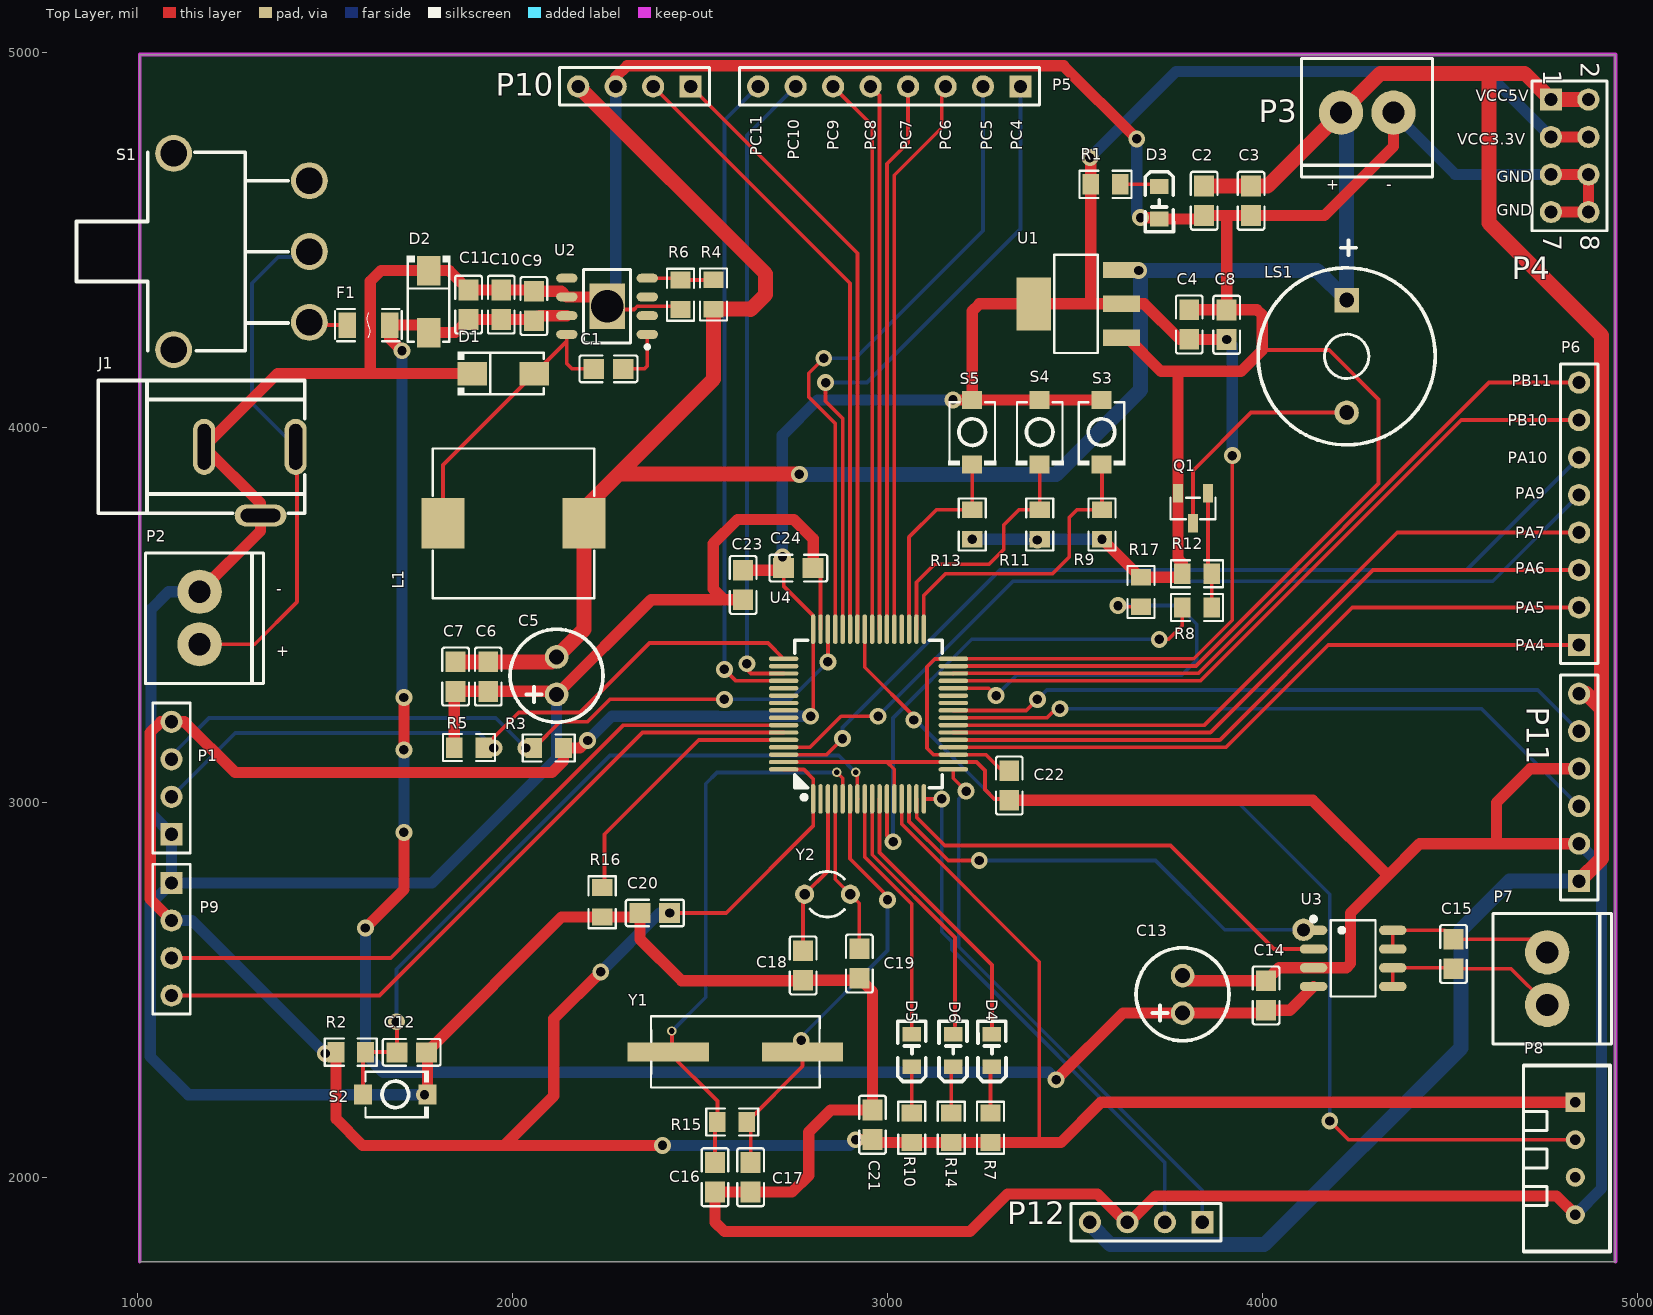
[diagram p0: Top Layer view]
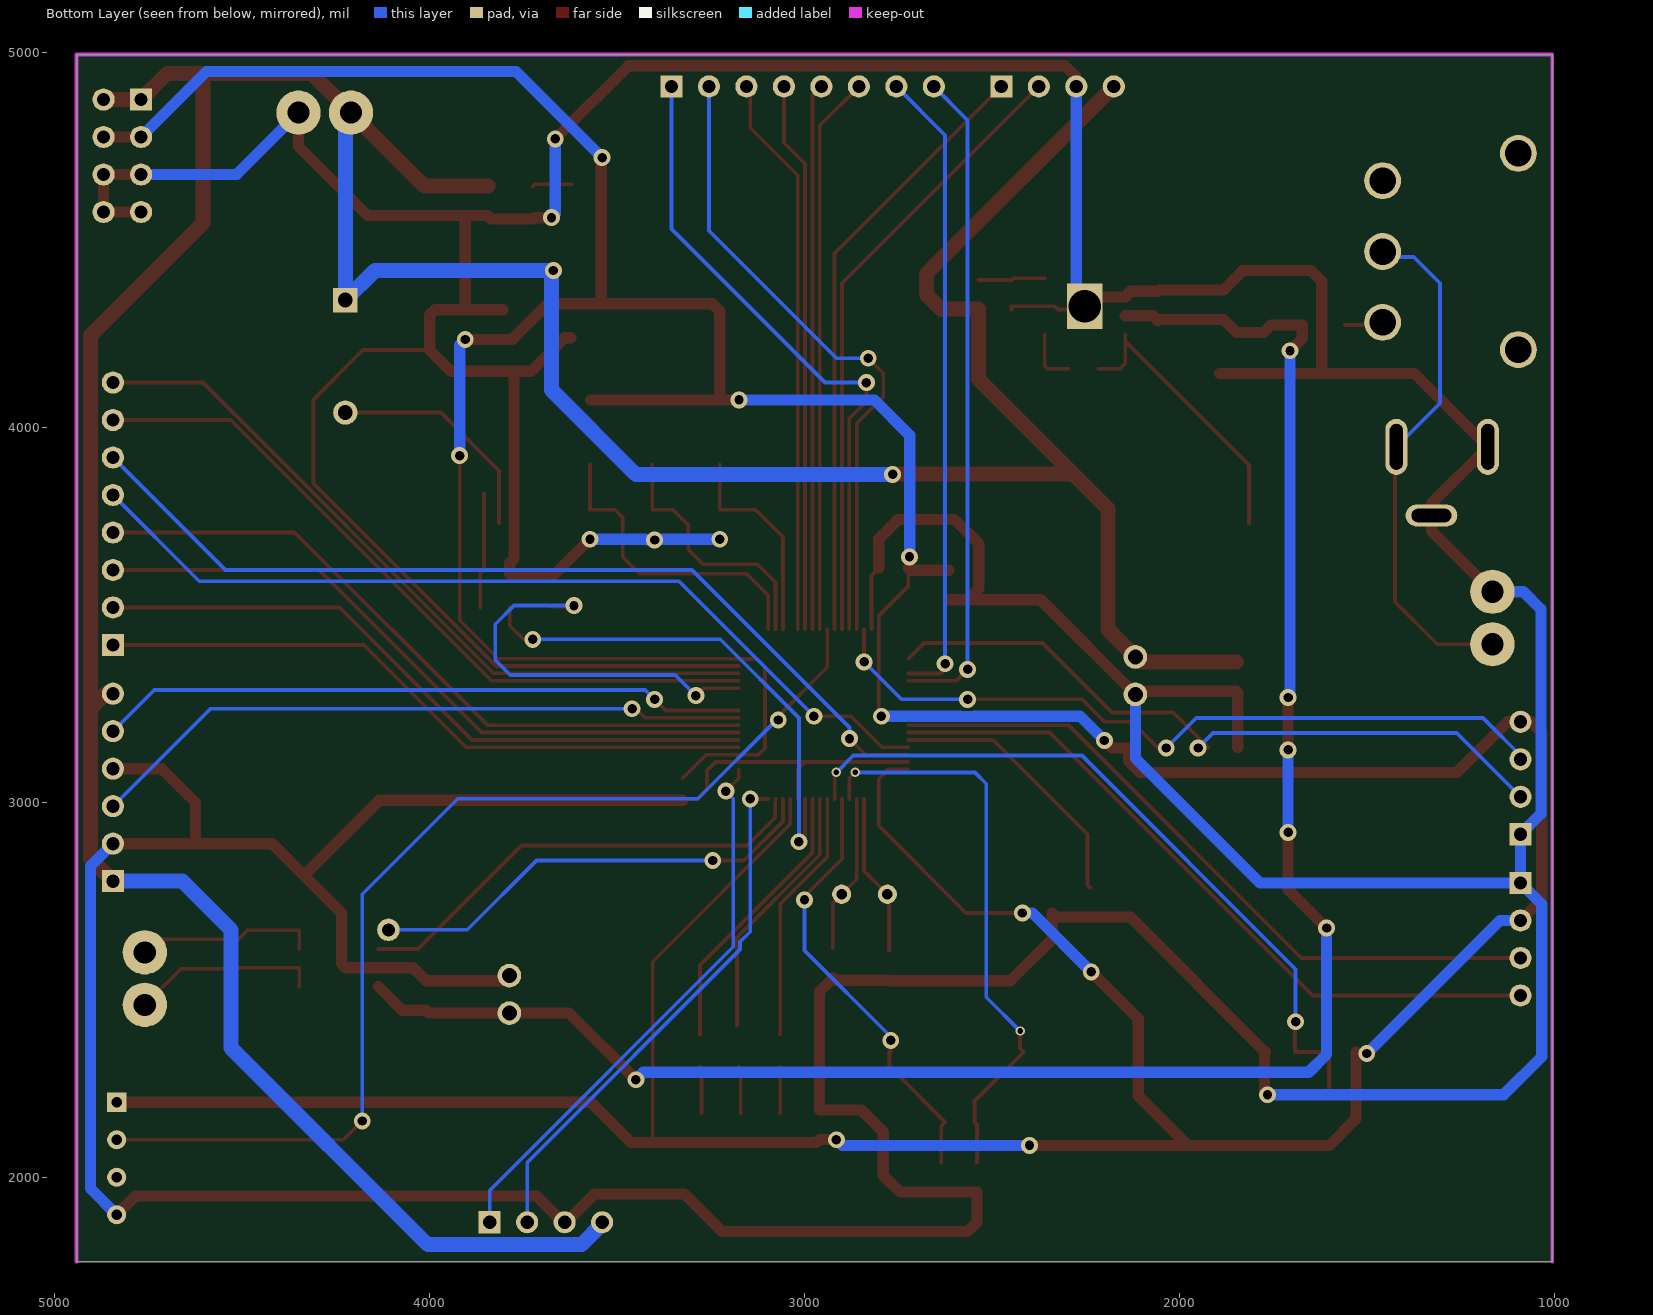
[diagram p1: Bottom Layer view, seen from below]
# Altium PCB MISC82341.PcbDoc
Units mil, origin at the board's own origin, x right, y up, seen from the top; angles counter-clockwise.
Board outline 3937.01 x 3220 mil, 2 copper layers (Top Layer, Bottom Layer); 75 components, 60 nets, 265 pads, 53 vias.

## Layer stack, top to bottom (the 12.6 mil dielectric is the usual default, probably not edited)
Top Solder: solder mask 0.4, Solder Resist, Dk 3.5
Top Layer: signal copper 1.4
Dielectric 1: dielectric 12.6, FR-4, Dk 4.8
Bottom Layer: signal copper 1.4
Bottom Solder: solder mask 0.4, Solder Resist, Dk 3.5

## Board outline
1005,1775 1005,4995 4942.01,4995 4942.01,1775

## Design rules (kind name [scope] priority, off if disabled: settings)
Clearance [All] p1: gap=8 ignorepadtopadclearanceinfootprint=FALSE except(7: SMDPad-SMDPad; 10: Arc-Fill Arc-Poly Arc-Region Track-Fill Track-Poly Track-Region THPad-Fill THPad-Poly THPad-Region Via-Fill Via-Poly Via-Region Fill-Fill Fill-Poly Fill-Region Poly-Poly Poly-Region Region-Region; 13: SMDPad-Fill SMDPad-Poly SMDPad-Region)
HoleSize [All] p1: absolutevalues=TRUE maxlimit=200 minlimit=1 maxpercent=80.000 minpercent=20.000
PolygonConnect [All] p1: connectstyle=Relief reliefconductorwidth=10 reliefentries=4 polygonreliefangle="90 Angle" airgapwidth=10
RoutingVias [All] p1: holewidth=20 width=30 viastyle="Through Hole" minholewidth=12 minwidth=24 maxholewidth=28 maxwidth=50
SolderMaskExpansion [All] p1: expansion=4
Width [All] p1: maxlimit=120 minlimit=8 preferedwidth=10
29 further rules are at their usual default settings.

## Components (designator, comment, footprint, x,y, rotation, side; value= is the part's Value field where it differs from the comment)
C1 "0.01uF" C0805 2255.63,4156.65 r180 top
C2 "10uF" C0805 3845,4605 r90 top
C3 "0.1uF" C0805 3970,4605 r90 top
C4 "10uF" C0805 3805,4275 r270 top
C5 "330uF/16V" 220uF 2110,3335 r90 top
C6 "0.1uF" C0805 1935,3335.63 r90 top
C7 "0.01uF" C0805 1847.84,3335.63 r90 top
C8 "0.1uF" C0805 3905,4274.37 r270 top
C9 "10uF/25V" C0805 2056.77,4324.17 r270 top
C10 "10uF/25V" C0805 1969.61,4327.91 r270 top
C11 "0.01uF" C0805 1882.45,4327.91 r270 top
C12 "0.1uF" C0805 1730.63,2333.33 r0 top
C13 "220uF/16V" 220uF 3780,2485 r90 top
C14 "0.01uF" C0805 4010,2485 r90 top
C15 "0.01uF" C0805 4510,2595.63 r90 top
C16 "22pF" C0805 2540,2000 r270 top
C17 "22pF" C0805 2635,2000 r270 top
C18 "15pF" C0805 2775,2565 r90 top
C19 "15pF" C0805 2925,2570 r270 top
C20 "0.1uF" C0805 2379.37,2705 r180 top
C21 "0.1uF" C0805 2960,2140 r90 top
C22 "0.1uF" C0805 3325,3045 r270 top
C23 "0.1uF" C0805 2615,3580 r270 top
C24 "0.1uF" C0805 2762.37,3625 r0 top
D1 "SS54" SMA 1975,4145 r0 top
D2 "SMBJ12A" SMA 1776.6,4336.74 r270 top
D3 "LED0" LED0805-RD_RED 3725,4600 r270 top
D4 "LED0" LED0805-RD_RED 3278.7,2338.31 r90 top
D5 "LED0" LED0805-RD_RED 3065,2338.31 r90 top
D6 "LED0" LED0805-RD_RED 3175,2338.31 r90 top
F1 "3A/16V" C70065 1611.93,4269.92 r0 top
J1 "DC-jack3" SANJIAO 1168.34,3957.44 r90 top
L1 "Inductor" DIANGAN 2005,3735 r180 top
LS1 "Speaker" BZ 4235,3805 r270 top
P1 "Header 4" HDR1X4 1090,2915 r90 top
P2 "Header 2" KF350 1165,3486.88 r180 top
P3 "Header 2" KF350 4275,4840 r90 top
P4 "Header 4X2" HDR2X4 4770,4875 r270 top
P5 "Header 8" HDR1X8 3355,4910 r180 top
P6 "Header 8" HDR1X8 4845,3420 r90 top
P7 "Header 2" KF350 4760,2525 r180 top
P8 "DHT11" DHT11 2528.78,-2097.7 r270 top
P9 "Header 4" HDR1X4 1090,2785 r270 top
P10 "HC-06" HDR1X4 2475,4910 r180 top
P11 "GP2Y1010AU0F" HDR1X6 4845,2790 r90 top
P12 "JW01" HDR1X4 3840,1880 r180 top
Q1 "NPN" QNPN 3815,3790 r90 top
R1 "10K" R0805 3580,4650 r180 top
R2 "10K" R0805 1566.41,2335.08 r180 top
R3 "10K" R0805 2094.58,3146.22 r180 top
R4 "10K" R0805 2534.78,4353.54 r270 top
R5 "10K" R0805 1885,3145 r0 top
R6 "3.16K" R0805 2449.01,4355.93 r90 top
R7 "10K" R0805 3273.78,2130.47 r270 top
R8 "1K" R0805 3827.19,3518.78 r0 top
R9 "10K" R0805 3571.06,3740 r270 top
R10 "10K" R0805 3063.78,2130.47 r270 top
R11 "10K" R0805 3405,3740 r270 top
R12 "10K" R0805 3827.19,3608.78 r0 top
R13 "10K" R0805 3225,3740 r270 top
R14 "10K" R0805 3168.78,2130.47 r270 top
R15 "1M" R0805 2584.07,2148.58 r180 top
R16 "10K" R0805 2240,2735 r90 top
R17 "10K" R0805 3675,3560 r270 top
S1 "SW-SPDT" SW-TH 1127.09,4463.54 r90 top
S2 "SW-PB" KAIGUAN 1685,2220 r0 top
S3 "SW-PB" KAIGUAN 3570,3990 r270 top
S4 "SW-PB" KAIGUAN 3405,3990 r270 top
S5 "SW-PB" KAIGUAN 3225,3990 r270 top
U1 "AMS1117" SOT-89 4700.81,4809.72 r0 top
U2 "TPS5450" CYF-SOIC-H 2252.01,4323.54 r180 top
U3 "RZ7889" SOP-8 4250,2580 r270 top
U4 "stm32f103r" LQFP-64 2945,3245 r0 top
Y1 "8MHz" JINGZHEN 2590,2335 r180 top
Y2 "32.768KHz" R38 2840,2755 r270 top

## Footprints (in the part's own frame and the unit in brackets; to place one, negate y for a bottom-side part, rotate by r counter-clockwise, add the part's x,y. Pads: shape width x height; smd on the part's side, far side on the other; paste and mask are expansions set on the pad)
220uF [mm]
  round 1.6 hole 1: 1(-1.193,-0.185) 2(1.347,-0.185)
  silkscreen extent -3.07,-3.33 3.23,2.96
BZ [mm]
  rect 1.65x1.65 hole 1: 1(-13.589,-0.254)
  round 1.65 hole 1: 2(-5.969,-0.254)
  silkscreen extent -17.65,-6.25 -3.78,5.75
C0805 [mm]
  rect 1.41x1.35 smd: 1(-1,0) 2(1,0)
  silkscreen extent -1.96,-0.9 1.96,0.9
C70065 [mil]
  rect 46.85x68.03 smd: 1(-53.62,3.62) 2(60.16,3.62)
  silkscreen extent -86,-39 93,47
CYF-SOIC-H [mm] "SOIC, 8-Leads, Body 4.90x3.90mm, Pitch 1.27mm, Thermal Pad 3.10x2.40mm, IPC Medium Density"
  oval 1.45x0.6 smd: 1(-2.725,1.905) 2(-2.725,0.635) 3(-2.725,-0.635) 4(-2.725,-1.905) 5(2.725,-1.905) 6(2.725,-0.635) 7(2.725,0.635) 8(2.725,1.905)
  rect 2.4x3.1 hole 2.2: 9(0,0)
  silkscreen extent -2.85,-2.5 1.6,2.88, body extent -2,-2.5 2,2.5, height 1.7
DHT11 [mil]
  rect 51x51 hole 28: 1(-4297.7,2306.22)
  round 51 hole 28: 2(-4197.7,2306.22) 3(-4097.7,2306.22) 4(-3997.7,2306.22)
  silkscreen extent -4396,2168 -3899,2399
DIANGAN [mm]
  rect 2.924x3.42 smd: 1(4.844,-0.241) 2(-4.712,-0.241)
  silkscreen extent -5.41,-5.32 5.54,4.84
HDR1X4 [mm] "Connector; Header; 4 Position"
  rect 1.5x1.5 hole 0.9: 1(0,0)
  round 1.5 hole 0.9: 2(2.54,0) 3(5.08,0) 4(7.62,0)
  silkscreen extent -1.27,-1.27 8.89,1.27
HDR1X6 [mm] "Connector; Header; 6 Position"
  rect 1.5x1.5 hole 0.9: 1(0,0)
  round 1.5 hole 0.9: 2(2.54,0) 3(5.08,0) 4(7.62,0) 5(10.16,0) 6(12.7,0)
  silkscreen extent -1.27,-1.27 13.97,1.27
HDR1X8 [mm] "Connector; Header; 8 Position"
  rect 1.5x1.5 hole 0.9: 1(0,0)
  round 1.5 hole 0.9: 2(2.54,0) 3(5.08,0) 4(7.62,0) 5(10.16,0) 6(12.7,0) 7(15.24,0) 8(17.78,0)
  silkscreen extent -1.27,-1.27 19.05,1.27
HDR2X4 [mm] "Connector; Header; 4x2 Position"
  rect 1.5x1.5 hole 0.9: 1(0,0)
  round 1.5 hole 0.9: 2(0,2.54) 3(2.54,0) 4(2.54,2.54) 5(5.08,0) 6(5.08,2.54) 7(7.62,0) 8(7.62,2.54)
  silkscreen extent -1.27,-1.27 8.89,3.81
JINGZHEN [mm]
  rect 5.5x1.3 smd: 1(-4.665,0.013) 2(4.441,0.013)
  silkscreen extent -5.83,-2.4 5.6,2.43
KAIGUAN [mm]
  rect 1.23x1.36 smd: 1(-2.13,0.027) 2(2.24,0.027)
  silkscreen extent -1.97,-1.59 2.31,1.64
KF350 [mm]
  round 3 hole 1.5: 1(0,-1.905) 2(0,1.651)
  silkscreen extent -4.34,-4.55 3.68,4.32
LED0805-RD_RED [mm]
  rect 1x1.25 smd: 1(-1.1,0) 2(1.1,0)
  silkscreen extent -2.1,-0.95 1.98,0.96
LQFP-64 [mm]
  oval 0.3x2 smd: 1(-3.639,-5.988) 2(-3.139,-5.988) 3(-2.639,-5.988) 4(-2.139,-5.988) 5(-1.639,-5.988) 6(-1.139,-5.988) 7(-0.639,-5.988) 8(-0.139,-5.988) 9(0.361,-5.988) 10(0.861,-5.988) 11(1.361,-5.988) 12(1.861,-5.988) 13(2.361,-5.988) 14(2.861,-5.988) 15(3.361,-5.988) 16(3.861,-5.988) 33(3.861,5.512) 34(3.361,5.512) 35(2.861,5.512) 36(2.361,5.512) 37(1.861,5.512) 38(1.361,5.512) 39(0.861,5.512) 40(0.361,5.512) 41(-0.139,5.512) 42(-0.639,5.512) 43(-1.139,5.512) 44(-1.639,5.512) 45(-2.139,5.512) 46(-2.639,5.512) 47(-3.139,5.512) 48(-3.639,5.512)
  oval 2x0.3 smd: 17(5.861,-3.988) 18(5.861,-3.488) 19(5.861,-2.988) 20(5.861,-2.488) 21(5.861,-1.988) 22(5.861,-1.488) 23(5.861,-0.988) 24(5.861,-0.488) 25(5.861,0.012) 26(5.861,0.512) 27(5.861,1.012) 28(5.861,1.512) 29(5.861,2.012) 30(5.861,2.512) 31(5.861,3.012) 32(5.861,3.512) 49(-5.639,3.512) 50(-5.639,3.012) 51(-5.639,2.512) 52(-5.639,2.012) 53(-5.639,1.512) 54(-5.639,1.012) 55(-5.639,0.512) 56(-5.639,0.012) 57(-5.639,-0.488) 58(-5.639,-0.988) 59(-5.639,-1.488) 60(-5.639,-1.988) 61(-5.639,-2.488) 62(-5.639,-2.988) 63(-5.639,-3.488) 64(-5.639,-3.988)
  silkscreen extent -4.89,-6.03 5.11,4.76
QNPN [mm]
  rect 1.25x0.7 smd: 1(-1.143,0) 2(0.889,-1.016) 3(0.889,1.016)
  silkscreen extent -0.88,-1.52 0.57,1.53
R38 [mm] "Crystal, Thru-Hole; 2 Leads; Body 3.1 x 8.2 mm (Dia.xH)"
  round 1.3 hole 0.7: 1(0,1.55) 2(0,-1.55)
  silkscreen extent -1.55,-1.19 1.55,1.17
R0805 [mil]
  rect 44.59x54.21 smd: 1(-40.93,1.22) 2(37.81,1.22)
  silkscreen extent -71,-35 68,37
SANJIAO [mm]
  oval 3.8x1.5 hole 0.9 slot 3.1 at 0 deg: 1(-0.226,-6.422) 2(-0.226,-0.222)
  oval 1.5x3.5 hole 0.9 slot 2.7 at 90 deg: 3(-4.876,-4.044)
  silkscreen extent -4.73,-7.04 4.27,6.96
SMA [mm]
  rect 2x1.593 smd: 1(-2.087,-0.023) 2(2.113,-0.023)
  silkscreen extent -3.09,-1.5 2.74,1.45
SOP-8 [mm]
  oval 0.63x1.865 smd: 1(-2.004,-2.878) 2(-0.734,-2.878) 3(0.536,-2.878) 4(1.806,-2.878) 5(1.806,2.487) 6(0.536,2.487) 7(-0.734,2.487) 8(-2.004,2.487)
  silkscreen extent -2.92,-3.03 2.48,1.33
SOT-89 [mm]
  rect 2.5x1.1 smd: 1(-27.355,-14.485) 2(-27.355,-12.185) 3(-27.355,-9.885)
  rect 2.34x3.6 smd: 2(-33.294,-12.185)
  silkscreen extent -31.9,-15.51 -28.95,-8.86
SW-TH [mm]
  round 2.5 hole 1.8: 1(-4.647,-8.402) 2(0.153,-8.402) 3(4.953,-8.402) 4(-6.497,0.798) 5(6.803,0.798)
  silkscreen extent -6.58,-6.98 6.88,7.37

## Part data
C1 C2 C3 C4 C5 C6 C7 C8 C9 C10 C11 C12 C13 C14 C15 C16 C17 C18 C19 C20 C21 C22 C23 C24: library part Cap, "Capacitor"
D1 D2: library part "D Schottky", "Schottky Diode"
D3 D4 D5 D6: "Typical INFRARED GaAs LED"
F1: library part "Fuse 1", "Fuse"
LS1: "Loudspeaker"
P1 P9: "Header, 4-Pin"
P2 P3 P7: "Header, 2-Pin"
P4: "Header, 4-Pin, Dual row"
P5 P6: "Header, 8-Pin"
P10 P12: library part "Header 4", "Header, 4-Pin"
P11: library part "Header 6", "Header, 6-Pin"
R1 R2 R3 R4 R5 R6 R7 R8 R9 R10 R11 R12 R13 R14 R15 R16 R17: library part Res2, "Resistor"
S1: "SPDT Subminiature Toggle Switch, Right Angle Mounting, Vertical Actuation"
S2 S3 S4 S5: "Switch"
Y1 Y2: library part XTAL, "Crystal Oscillator"

## Free pads (board coordinates)
  round 60 hole 35: 3(4110,2660)

## Via types
v1: diameter 45, hole 25, Top Layer to Bottom Layer, 50 vias
v2: diameter 25, hole 15, Top Layer to Bottom Layer, 3 vias

## Nets (pads, with @x,y where several pads share a name; then routed paths per layer and width w, separated by ;. In a path a pad name is that pad's centre, name@x,y a point inside that pad or via, vN(x,y) a via of type N, cw(c..) or ccw(c..) an arc to the next point about the centre after c; other vN are vias at no path point)
B: D4.2 U4.10 | length 751.8
  Top Layer w10: U4.10 2978.91,2866.09 3278.7,2566.3 D4.2
BEEP: R8.1 U4.11 | length 1373.1
  Top Layer w10: U4.11 2998.59,2911.41 v1(3015,2895) ; v1(3725,3435) 3750,3435 3786.26,3471.26 R8.1
  Bottom Layer w10: v1(3015,2895) 3015,3225 3225,3435 v1(3725,3435)
"CAN RX": P5.1 U4.44 | length 1746.9
  Top Layer w10: v1(2835,4120) 2835,4070 2880.48,4024.52 U4.44
  Bottom Layer w10: v1(2835,4120) 2945.48,4120 3355,4529.52 P5.1
"CAN TX": P5.2 U4.45 | length 1719.7
  Top Layer w10: v1(2830,4185) 2790,4145 2790,4081.74 2860.8,4010.94 U4.45
  Bottom Layer w10: v1(2830,4185) 2915,4185 3255,4525 P5.2
DATA: P8.2 U4.41 | length 2893.5
  Top Layer w10: U4.41 2939.54,3360.46 3080,3220 v1(3070,3220) ; v1(4180,2150) 4230,2100 P8.2
  Bottom Layer w10: v1(3070,3220) 3075,3220 3285,3010 3925,3010 4180,2755 v1(4180,2150)
"DC IN": C9.2 C10.2 C11.2 C13.1 C14.1 D2.2 F1.2 U2.7 U3.4 | length 5155.2
  Top Layer w30: v1(1607.35,2665) 1710,2767.65 v1(1710,2920) ; v1(1705,4205) 1672.09,4237.91 F1.2 1755.7,4273.54 D2.2 1847.45,4253.54 C11.2 C10.2 2053.03,4288.54 C9.2 2070.51,4298.54 U2.7 ; v1(1710,3140) v1(1710,3280) ; v1(3450,2260) 3628.02,2438.02 C13.1 4002.39,2438.02 C14.1 4073.46,2445.63 U3.4
  Bottom Layer w30: v1(1607.35,2665) 1607.35,2327.65 1655,2280 3430,2280 v1(3450,2260) ; v1@1705,3290 v1(1705,4205) ; v1(1710,2920) v1(1710,3140)
G: D6.2 U4.9 | length 695.7
  Top Layer w10: U4.9 2959.22,2860.33 3180,2639.54 3180,2405
GND: C2.1 C3.1 C4.1 C5.1 C6.1 C7.1 C8.1 C9.1 C10.1 C11.1 C12.2 C13.2 C14.2 C16.2 C17.2 C18.1 C19.2 C20.2 C21.2 C22.2 C23.2 C24.2 D1.1 D2.1 D3.2 J1.2 J1.3 P1.1 P2.1 P3.1 P4.5 P4.6 P4.7 P4.8 P8.4 P9.1 P10.3 P11.2 P11.4 P12.3 Q1.3 R5.1 R6.1 R9.2 R11.2 R12.1 R13.2 R16.1 R17.1 S2.2 U1.1 U2.6 U2.9 U3.3 U4.12 U4.18 U4.31 U4.47 U4.63 | length 25294.4
  Top Layer w10: U2.9 2260.55,4315 2323.94,4315 2332.28,4323.35 2447.78,4323.35 R6.1 ; U4.63 2999.03,3107.69 ; C24.2 2821.43,3605.31 U4.47 ; U4.12 3018.28,3088.44 2999.03,3107.69 ; U4.31 3823.13,3363.59 4310,3850.46 4310,4075 4178.35,4206.65 4000,4206.65 ; C22.2 3321.36,3009.27 3285,3009.27 3260,3034.27 3260,3085 3237.31,3107.69 U4.18 2999.03,3107.69
  Top Layer w30: P2.1 1327.57,3724.45 J1.3 1327.57,3798.06 J1.2 1372.65,4144.1 1620,4144.1 ; S2.2 1773.2,2330.13 C12.2 2130.74,2694.07 R16.1 2329.07,2694.07 C20.2 2340,2635 2450.63,2524.37 2773.74,2524.37 C18.1 2920,2525.63 C19.2 2960,2495.63 C21.2 2848.74,2179.37 2790,2120.63 2790,2005 2745.63,1960.63 C17.2 C16.2 2540,1880 2565,1855 3220,1855 3320,1955 3560,1955 3640,1875 3715,1950 4785,1950 P8.4 ; R5.1 1844.07,3292.49 C7.1 C6.1 2109.05,3296.26 C5.1 2369.9,3540.63 2564.37,3540.63 ; D1.1 1620,4144.1 ; U2.9 2227.01,4348.54 U2.6 2129.73,4363.54 C9.1 2053.03,4367.28 C10.1 C11.1 1830.83,4418.9 D2.1 1648.9,4418.9 1620,4390 1620,4144.1 ; P10.3 2275,4935 2305,4965 3470,4965 v1@3660,4775 ; C23.2 2564.37,3540.63 ; C24.2 2801.74,3703.26 2750,3755 2600,3755 2535,3690 2535,3570 2564.37,3540.63 ; C22.2 4134.37,3005.63 4335,2805 ; v1(3572.29,3702.19) 3673.55,3600.93 R17.1 3777.19,3600.93 R12.1 3786.26,3638.74 3775,3650 Q1.3 3775,4145 3770,4150 ; U1.1 3640.55,4239.45 3730,4150 3770,4150 ; v1(3675,4560) 3721.7,4560 D3.2 3836.06,4556.69 C2.1 3900,4565.63 ; C13.2 3800.94,2524.37 C14.2 4044.51,2558.88 U3.3 4223.88,2558.88 4235,2570 4235,2705 4335,2805 ; C4.1 C8.1@3905,4314.37 ; P3.1 4350,4750 4165.63,4565.63 C3.1 3900,4565.63 ; P4.7 P4.8 P4.6 P4.5 ; P11.2 4625,2890 ; P11.4 4715,3090 4625,3000 4625,2890 ; 3770,4150 3943.35,4150 4000,4206.65 4000,4300 3985,4315 3984.37,4314.37 C8.1@3905,4314.37 ; 3900,4565.63 3905,4560.63 C8.1@3905,4314.37 ; 4335,2805 4420,2890 4625,2890
  Bottom Layer w30: P9.1@1080,2785 1090,2795 P1.1 1035,2970 1035,3515 1081.88,3561.88 P2.1 ; v1(1765,2220) 1135,2220 1033,2322 1033,2728 P9.1 1785,2785 2117.29,3117.29 C5.1 ; U2.9 2275,4346.53 P10.3 ; v1(3226.22,3702.19) v1@3400,3702.19 ; v1(3400,3700) 3422.81,3700 3425,3702.19 v1(3572.29,3702.19) ; v1(3665,4770) 3665,4570 v1(3675,4560) ; P3.1 4515,4675 P4.5 ; P8.4 4905,1970 4905,2830 P11.2
NetC1_1: C1.1 U2.1 | length 151.7
  Top Layer w10: C1.1 2351.65,4156.65 2359.29,4164.29 U2.1
NetC1_2: C1.2 D1.2 L1.1 U2.8 | length 778.5
  Top Layer w10: L1.1 1814.28,3900.18 D1.2 2144.73,4230.62 ; U2.8 2144.73,4230.62 ; C1.2 2158.35,4156.65 2144.73,4170.27 2144.73,4230.62
NetC15_1: C15.1 P7.2 U3.5 U3.6 | length 503
  Top Layer w10: U3.5 U3.6 4507.38,2558.88 C15.1 4663.74,2556.26 P7.2
NetC15_2: C15.2 P7.1 U3.7 U3.8 | length 486.5
  Top Layer w10: U3.7 U3.8 4486.12,2658.88 C15.2 4725,2635 P7.1
NetC16_1: C16.1 R15.2 U4.5 Y1.2 | length 1548.4
  Top Layer w10: v2(2425,2390) 2425,2344.3 Y1.2 2546.26,2203.39 R15.2 2540,2141.1 C16.1 ; v2(2865,3080) 2880.48,3064.52 U4.5
  Bottom Layer w10: v2(2425,2390) 2515,2480 2515,3050 2545,3080 v2(2865,3080)
NetC17_1: C17.1 R15.1 U4.6 Y1.1 | length 1172.7
  Top Layer w10: C17.1 2635,2137.36 R15.1 2773.67,2296.03 Y1.1 2770.52,2334.48 2770,2335 v1(2770,2365) ; U4.6 2900.17,2849.83 v1@3005,2745
  Bottom Layer w10: v1(2770,2365) 2770,2375 3000,2605 v1(3000,2740)
NetC18_2: C18.2 U4.3 Y2.2 | length 432.3
  Top Layer w10: C18.2 2775,2751.02 Y2.2 2841.11,2817.13 U4.3
NetC19_1: C19.1 U4.4 Y2.1 | length 426.5
  Top Layer w10: U4.4 2860.8,2795.22 Y2.1 2925,2731.02 C19.1
NetD3_1: D3.1 R1.1 | length 106.3
  Top Layer w10: R1.1 3719.54,4648.78 D3.1
NetD4_1: D4.1 R7.1 | length 125.1
  Top Layer w10: R7.1 3275,2291.3 D4.1
NetD5_1: D5.1 R10.1 | length 123.6
  Top Layer w10: R10.1 D5.1
NetD6_1: D6.1 R14.1 | length 125.7
  Top Layer w10: R14.1 3170,2290 D6.1
NetF1_1: F1.1 S1.1 | length 103.4
  Top Layer w10: S1.1 1464.91,4273.54 F1.1
NetJ1_1: J1.1 P2.2 S1.2 | length 1394.5
  Top Layer w10: P2.2 1311.88,3421.88 1425,3535 1425,3944.73 J1.1
  Bottom Layer w10: J1.1 1305,4064.73 1305,4385 1375,4455 1443.31,4455 S1.2
NetLS1_2: LS1.2 Q1.1 | length 614.2
  Top Layer w10: Q1.1 3815,3885 3970,4040 LS1.2
NetQ1_2: Q1.2 R8.2 R12.2 | length 309.1
  Top Layer w10: Q1.2 3855,3620 R12.2 R8.2
NetR4_1: R4.1 R6.2 U2.4 | length 179
  Top Layer w10: U2.4 2442.98,4398.54 R6.2 2535.27,4393.74 R4.1
NetR16_2: R16.2 U4.60 | length 727.1
  Top Layer w10: R16.2 2245,2779.03 2245,2915 2496.74,3166.74 U4.60
NetR17_2: R17.2 U4.28 | length 1084.8
  Top Layer w10: U4.28 3270.46,3304.54 v1(3290,3285) ; v1(3615,3525) 3617.81,3522.19 R17.2
  Bottom Layer w10: v1(3290,3285) 3345,3340 3785,3340 3825,3380 3825,3475 3775,3525 v1(3615,3525)
PA0: pad.3 U3.1 U4.14 | length 1227.1
  Top Layer w10: U4.14 3057.65,2949.37 3162.02,2845 v1@3240,2845
  Bottom Layer w10: v1(3245,2845) 3715,2845 3900,2660 pad.3
PA1: U3.2 U4.15 | length 1253.9
  Top Layer w10: U4.15 3078.11,3008.49 3078.11,2959.6 3152.71,2885 3755,2885 4031.12,2608.88 U3.2
PA2: P12.2 U4.16 | length 1428.7
  Top Layer w10: U4.16 v1(3145,3009.27)
  Bottom Layer w10: v1(3145,3009.27) 3145,2655 3172,2628 3172,2607.54 3740,2039.54 P12.2 P12.2@3740,1875
PA3: P12.1 U4.17 | length 1504.7
  Top Layer w10: U4.17 3175.75,3064.25 v1(3210,3030)
  Bottom Layer w10: v1(3210,3030) 3190,3010 3190,2615 3840,1965 P12.1 P12.1@3840,1875
PA4: P6.1 U4.20 | length 1782.3
  Top Layer w10: U4.20 3902.84,3147.06 4175.78,3420 P6.1
PA5: P6.2 U4.21 | length 1815.6
  Top Layer w10: U4.21 3886.74,3166.74 4240,3520 P6.2
PA6: P6.3 U4.22 | length 1848.8
  Top Layer w10: U4.22 3861.43,3186.43 4295,3620 P6.3
PA7: P6.4 U4.23 | length 1882.1
  Top Layer w10: U4.23 3846.11,3206.11 4360,3720 P6.4
PA9: P10.1 U4.42 | length 1632.3
  Top Layer w10: P10.1 2919.85,4465.15 U4.42
PA10: P10.2 U4.43 | length 1665.5
  Top Layer w10: P10.2 2900.17,4384.83 U4.43
PB6: P9.3 U4.58 | length 1900.3
  Top Layer w10: P9.3@1080,2585 P9.3 1675,2585 2296.11,3206.11 U4.58
PB7: P9.4 U4.59 | length 1933.5
  Top Layer w10: P9.4@1080,2485 P9.4 1645,2485 2346.43,3186.43 U4.59
PB8: P6.5 U4.61 | length 2400.7
  Top Layer w10: U4.61 2793.49,3147.06 2876.43,3230 v1(2975,3230)
  Bottom Layer w10: v1(2975,3230) 3335,3590 4615,3590 P6.5
PB9: P6.6 U4.62 | length 2467.9
  Top Layer w10: U4.62 2837.37,3127.37 v1(2880,3170)
  Bottom Layer w10: v1(2880,3170) 2880,3200 3300,3620 4545,3620 P6.6
PB10: P6.7 U4.29 | length 1957.5
  Top Layer w10: U4.29 3834.68,3324.22 4530.46,4020 P6.7
PB11: P6.8 U4.30 | length 1990.7
  Top Layer w10: U4.30 3176.52,3344.68 3829.68,3344.68 4605,4120 P6.8
PB12: R9.1 S3.2 U4.33 | length 843
  Top Layer w10: U4.33 3097.02,3552.02 3155,3610 3440,3610 3485,3655 3485,3760 3505.93,3780.93 R9.1 3572.29,3900.58 S3.2
PB13: R11.1 S4.2 U4.34 | length 693.4
  Top Layer w10: U4.34 3077.33,3587.33 3125,3635 3270,3635 3310,3675 3310,3740 3350.93,3780.93 R11.1 3406.22,3901.64 S4.2
PB14: R13.1 S5.2 U4.35 | length 565.5
  Top Layer w10: U4.35 3057.65,3707.65 3130.93,3780.93 R13.1 3226.22,3901.64 S5.2
PC4: P11.3 U4.24 | length 1787
  Top Layer w10: U4.24 3425.8,3225.8 3450,3250 v1(3460,3250)
  Bottom Layer w10: v1(3460,3250) 4585,3250 P11.3
PC5: P11.5 U4.25 | length 1737.4
  Top Layer w10: U4.25 3370.48,3245.48 v1(3400,3275)
  Bottom Layer w10: v1(3400,3275) 3425,3300 4735,3300 P11.5
PC6: P5.3 U4.37 | length 1504.6
  Top Layer w10: U4.37 3018.28,4673.28 3145,4800 3145,4900 P5.3
PC7: P5.4 U4.38 | length 1471.4
  Top Layer w10: U4.38 2998.59,4703.59 3055,4760 P5.4
PC8: P5.5 U4.39 | length 1457.9
  Top Layer w10: P5.5 2978.91,4886.09 U4.39
PC9: P5.6 U4.40 | length 1491.2
  Top Layer w10: P5.6 2959.22,4805.78 U4.40
PC10: P5.7 U4.51 | length 1703.5
  Top Layer w10: v1@2620,3360 2636.09,3343.91 U4.51
  Bottom Layer w10: v1(2625,3370) 2625,4780 P5.7
PC11: P5.8 U4.52 | length 1763
  Top Layer w10: v1(2565,3355) 2595.78,3324.22 U4.52
  Bottom Layer w10: v1(2565,3355) 2565,4820 P5.8
R: D5.2 U4.8 | length 679.6
  Top Layer w10: U4.8 2939.54,2854.55 3065,2729.09 D5.2
RESET: C12.1 R2.1 S2.1 U4.7 | length 1974.2
  Top Layer w10: S2.1 1601.16,2327.67 R2.1 1690.73,2333.86 C12.1 1691.26,2413.74 v1(1690,2415) ; v2(2915,3080) 2919.07,3075.93 2919.07,3010.04 U4.7
  Bottom Layer w10: v1(1690,2415) 1690,2555 2260,3125 2870,3125 v2(2915,3080)
SWCLK: P1.2 R5.2 U4.49 | length 1889.9
  Top Layer w10: R5.2 2016.58,3240 2180,3240 2365,3425 2681.29,3425 U4.49
  Bottom Layer w10: P1.2@1080,3015 P1.2 1260,3185 1910,3185 v1(1950,3145)
SWDIO: P1.3 R3.2 U4.46 | length 2008.1
  Top Layer w10: R3.2 2126.77,3215 2200,3215 2260,3275 v1(2565,3275) ; v1(2841.11,3375) U4.46
  Bottom Layer w10: P1.3@1085.5,3109.5 1080,3115 1190,3225 1955,3225 v1(2035,3145) ; v1(2565,3275) 2741.11,3275 v1(2841.11,3375)
VCC3.3V: C4.2 C8.2 C20.1 C21.1 C22.1 C23.1 C24.1 P1.4 P4.3 P4.4 P8.1 P9.2 R1.2 R2.2 R3.1 R7.2 R10.2 R14.2 S3.1 S4.1 S5.1 U1.2 U4.1 U4.13 U4.19 U4.32 U4.48 U4.64 | length 15873.1
  Top Layer w10: v1(2418.74,2705) 2570,2705 2801.74,2936.74 U4.1 2801.74,3063.26 2777,3088 U4.64 ; C24.1 2723,3577 2801.74,3498.26 U4.48 2801.74,3236.74 v1(2795,3230) ; U4.13 3037.96,2942.04 3405,2575 3405,2092.66 ; C22.1@3325,3065 3262.63,3127.37 U4.19 3122.63,3127.37 3105.5,3144.5 3105.5,3361.92 3126.08,3382.5 3174.96,3382.5 U4.32 3817.37,3383.28 3920,3485.91 v1(3920,3925)
  Top Layer w30: P9.2 1033,2742 1033,3186.43 1061.57,3215 P1.4 1125,3215 1260,3080 2105,3080 2135.51,3110.51 R3.1 2180,3145 v1(2200,3165) ; v1(1500,2330) 1524.75,2330 R2.2 1528.61,2156.39 1600,2085 1977.64,2085 ; v1(2235,2547.99) 2110,2422.99 2110,2217.36 1977.64,2085 ; v1(2400,2085) 1977.64,2085 ; C23.1 2717.37,3619.37 C24.1 ; v1(2915,2100) 2915.63,2100.63 C21.1 2967.97,2092.66 R10.2 R14.2 R7.2 3405,2092.66 3462.66,2092.66 3570,2200 P8.1 ; v1(3175,4073.84) S5.1 ; v1(3540,4720) 3542.19,4717.81 R1.2 3542.19,4330 ; S3.1 S4.1 S5.1 ; v1(3905,4235) 3780,4235 3685,4330 3623.85,4330 3542.19,4330 ; P4.3 P4.4 ; S5.1 3226.06,4311.06 3245,4330 3390,4330 3542.19,4330
  Bottom Layer w30: P9.2 1145,2685 v1(1500,2330) ; v1(2200,3165) 2265,3230 2545.65,3230 2546.15,3229.5 2583.85,3229.5 2584.35,3230 v1(2795,3230) ; v1(2235,2547.99) 2392.01,2705 v1(2418.74,2705) ; v1(2400,2085) 2900,2085 v1(2915,2100) ; v1(2720,3655) 2719.5,3655.5 2719.5,3979.5 2813.84,4073.84 v1(3175,4073.84) ; v1(3540,4720) 3770,4950 4595,4950 P4.3 ; v1(3905,4235) 3920,4220 v1(3920,3925)
VCC5V: C2.2 C3.2 C5.2 C6.2 C7.2 L1.2 LS1.1 P3.2 P4.1 P4.2 P10.4 P11.1 P11.6 P12.4 R4.2 U1.3 | length 10667.4
  Top Layer w40: C7.2 C6.2 2104.27,3375 C5.2 2190.5,3461.24 L1.2 2190.5,3783.5 2283.5,3876.5 ; P10.4 2675,4410 2675,4355 2635,4315 2634.27,4315.73 R4.2 2536,4129 2283.5,3876.5 ; v1(2765,3875) 2763.5,3876.5 2283.5,3876.5 ; C2.2 C3.2 4014.37,4644.37 P3.2 4315,4945 4605,4945 ; P11.1 4905,2850 4905,3250 ; P11.6 4865,3290 4905,3250 ; P4.2 P4.1 4700,4945 4605,4945 ; 4605,4945 4605,4545.55 4905,4245.55 4905,3250
  Bottom Layer w40: v1(2765,3875) 3450,3875 3675,4100 3675,4413.9 v1(3670,4418.9) 4146.1,4418.9 LS1.1 4225,4825 P3.2 ; P12.4@3540,1875 3595,1820 4005,1820 4530,2345 4530,2660 4660,2790 P11.1
pads on no net: P8.3 S1.3 S1.4 S1.5 U2.2 U2.3 U2.5 U4.2 U4.26 U4.27 U4.36 U4.50 U4.53 U4.54 U4.55 U4.56 U4.57

## Polygon pours and split planes (outlines as drawn)
no net on Top Layer "NONET_L01_P001" (solid, remove dead copper, pour order 1): 1120,5085
GND on Top Layer "GND_L01_P004" (solid, pour order 4): 1000,5000

## Keep-outs
Keep-Out Layer:
  lines w10: 1005,1775 1005,4995 4942.01,4995 4942.01,1775

## Silkscreen, mask and mechanical layers (free items; w line width, h text height)
Top Overlay:
  text "VCC5V" at 4570,4870 h30
  text "VCC3.3V" at 4520,4755 h30
  text "PC9" at 2870,4740 h30 r90
  text "PC8" at 2970,4740 h30 r90
  text "PC7" at 3065,4740 h30 r90
  text "PC6" at 3170,4740 h30 r90
  text "PC5" at 3280,4740 h30 r90
  text "PC4" at 3360,4740 h30 r90
  text "PC11" at 2665,4725 h30 r90
  text "PC10" at 2765,4715 h30 r90
  text "GND" at 4625,4655 h30
  text "+" at 4170,4635 h30
  text "-" at 4330,4635 h30
  text "GND" at 4625,4565 h30
  text "PB11" at 4665,4110 h30
  text "PB10" at 4655,4005 h30
  text "PA10" at 4655,3905 h30
  text "PA9" at 4675,3810 h30
  text "PA7" at 4675,3705 h30
  text "PA6" at 4675,3610 h30
  text "-" at 1370,3555 h30
  text "PA5" at 4675,3505 h30
  text "PA4" at 4675,3405 h30
  text "+" at 1370,3390 h30
Drill Drawing:
  lines w7.99: 1005,1775 4942.01,1775